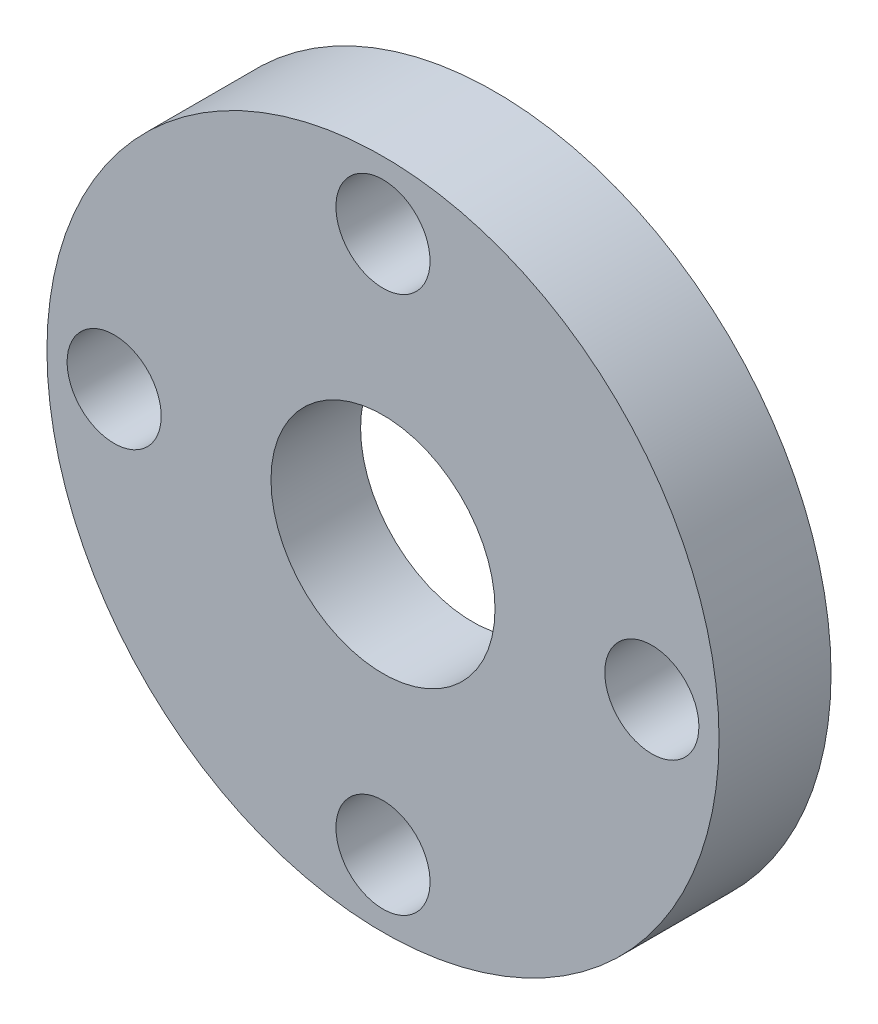
SolidWorks part; units mm, degrees
material "316L"
ref_plane "Front Plane" through (0, 0, 0) normal (0, 0, 1) x (1, 0, 0)
ref_plane "Top Plane" through (0, 0, 0) normal (0, 1, 0) x (1, 0, 0)
ref_plane "Right Plane" through (0, 0, 0) normal (1, 0, 0) x (0, 0, -1)
sketch "Sketch1" plane through (0, 0, 0) normal (0, 0, 1) x (1, 0, 0)
  circle A0 centre (0, 0) radius 15
  dimension "D1" = 30
extrude "Boss-Extrude1" add sketch "Sketch1" along normal blind 5
sketch "Sketch2" plane through (0, 0, 5) normal (0, 0, 1) x (1, 0, 0)
  circle A0 centre (0, 12) radius 2.1
  dimension "D1" = 12
  dimension "D2" = 4.2
extrude "Cut-Extrude1" cut sketch "Sketch2" against normal through all
pattern_circular "CirPattern1" count 4 over 360 about axis through (0, 0, 0) along (0, 0, 1) of "Cut-Extrude1"
sketch "Sketch3" plane through (0, 0, 0) normal (0, 0, -1) x (-1, 0, 0)
  circle A0 centre (0, 0) radius 8
  dimension "D1" = 16
extrude "Cut-Extrude2" cut sketch "Sketch3" against normal blind 1
sketch "Sketch4" plane through (0, 0, 5) normal (0, 0, 1) x (1, 0, 0)
  circle A0 centre (0, 0) radius 5
  dimension "D1" = 10
extrude "Cut-Extrude3" cut sketch "Sketch4" against normal through all
chamfer "Chamfer1" [suppressed] distance 1.5 angle 45
